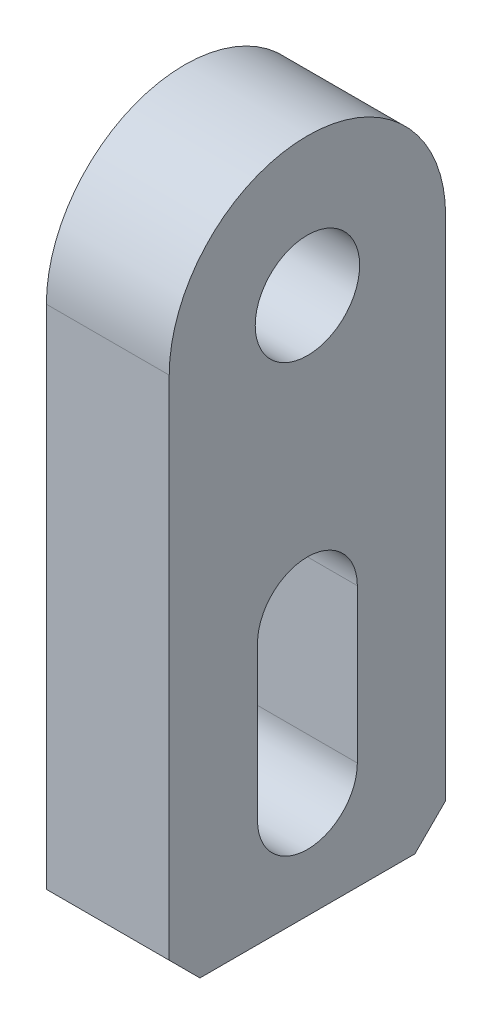
SolidWorks part; units mm, degrees
material "S45C"
ref_plane "Front Plane" through (0, 0, 0) normal (0, 0, 1) x (1, 0, 0)
ref_plane "Top Plane" through (0, 0, 0) normal (0, 1, 0) x (1, 0, 0)
ref_plane "Right Plane" through (0, 0, 0) normal (1, 0, 0) x (0, 0, -1)
sketch "Sketch1" plane through (0, 0, 0) normal (1, 0, 0) x (0, 0, -1)
  line L0 (0, -21.0636) -> (0, 121.0464) construction
  line L1 (-9, 0) -> (9, 0)
  line L2 (-9, 0) -> (-9, 35)
  line L3 (0, 17) -> (0, 7) construction
  line L4 (9, 0) -> (9, 35)
  line L5 (3.25, 17) -> (3.25, 7)
  line L6 (-3.25, 17) -> (-3.25, 7)
  arc A0 (9, 35) -> (-9, 35) centre (0, 35) ccw
  arc A1 (3.25, 17) -> (-3.25, 17) centre (0, 17) ccw
  arc A2 (-3.25, 7) -> (3.25, 7) centre (0, 7) ccw
  point P10 (0, 12)
  dimension "D3" = 3.25
  dimension "D1" = 18
  dimension "D2" = 35
  dimension "D4" = 12
  dimension "D5" = 10
extrude "Boss-Extrude1" add sketch "Sketch1" along normal mid plane 8
hole_wizard "M8 Tapped Hole1" positions "Sketch3" profile "Sketch2" tap size "M8" standard "Gb"
sketch "Sketch3" plane through (-4, 0, 0) normal (-1, 0, 0) x (0, 0, 1)
  point P0 (0, 35)
sketch "Sketch2" plane through (-4, 35, 0) normal (0, 1, 0) x (0, 0, 1)
  line L0 (0, 0) -> (0, 24.2929)
  line L1 (0, 24.2929) -> (3.4, 22.25)
  line L2 (3.4, 22.25) -> (3.4, 0)
  line L5 (3.4, 0) -> (0, 0)
  line L10 (0, 24.2929) -> (-3.4, 22.25) construction
  line L11 (0, -6.35) -> (0, 107.95) construction
  dimension "螺纹孔钻头直径" = 6.8
  dimension "螺纹孔钻头深度" = 22.25
  dimension "导头角度" = 118
cosmetic thread "Cosmetic Thread1" parameters "D1"=12, "D2"=8
chamfer "Chamfer1" distance 2 angle 45 2 edges at (0, 0, 9) (0, 0, -9)
